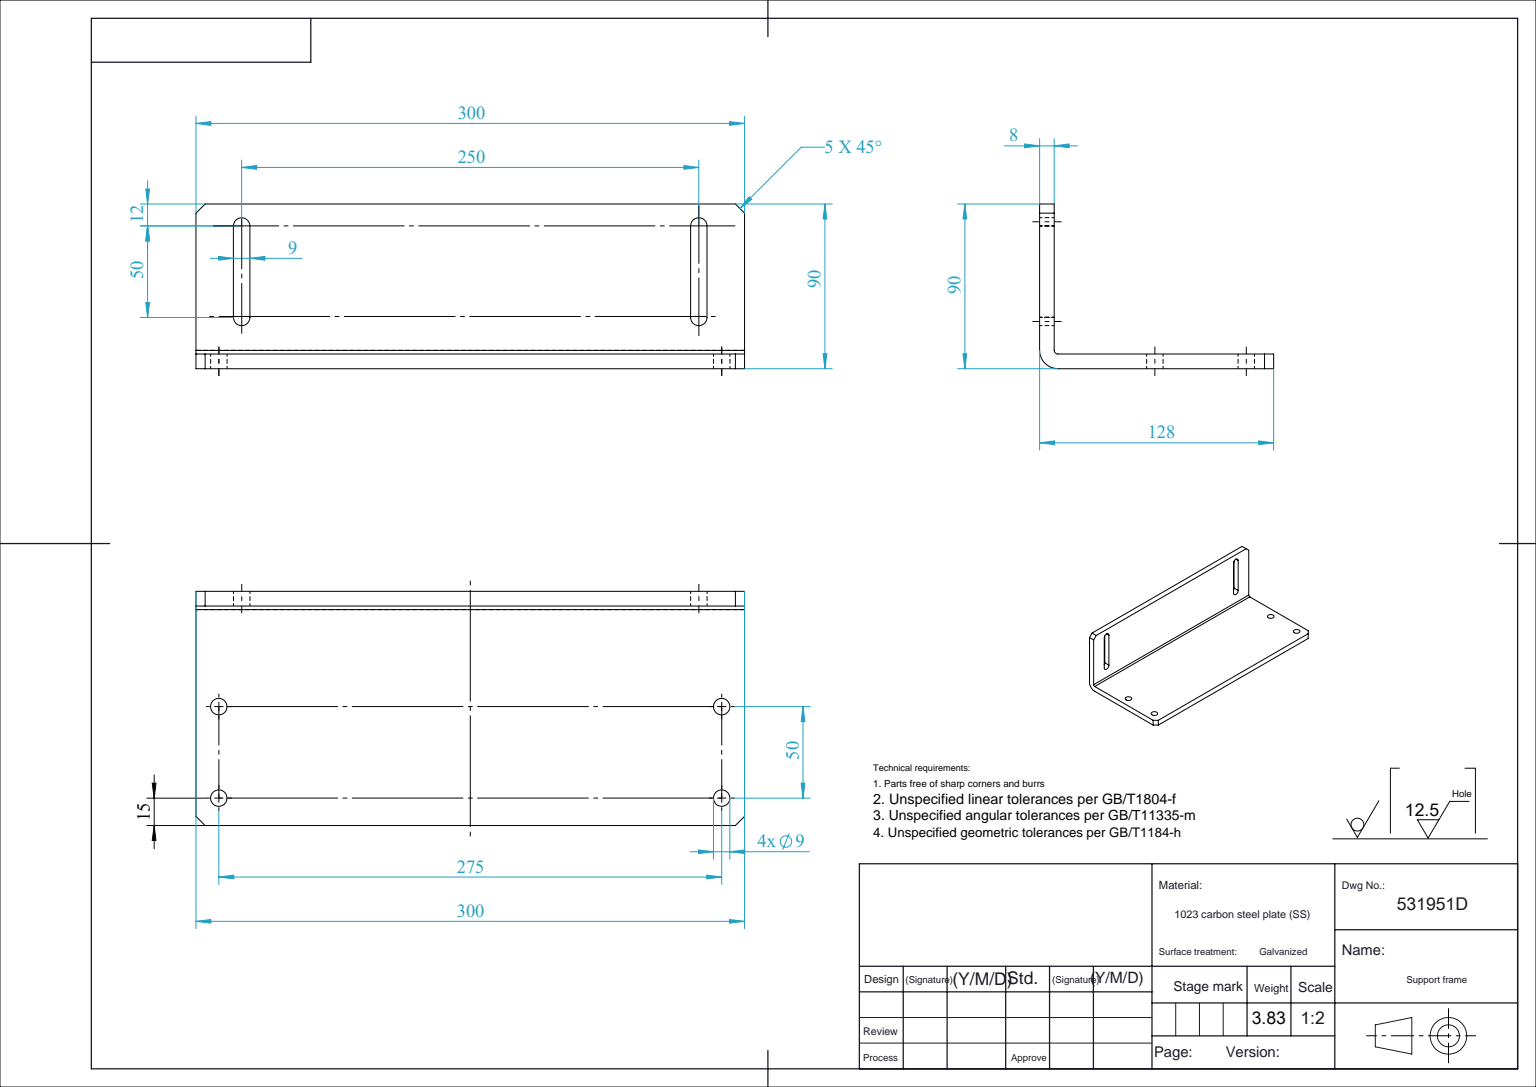
SolidWorks part; units mm, degrees
material "1023 carbon steel plate (SS)"
ref_plane "Front Plane" through (0, 0, 0) normal (0, 0, 1) x (1, 0, 0)
ref_plane "Top Plane" through (0, 0, 0) normal (0, 1, 0) x (1, 0, 0)
ref_plane "Right Plane" through (0, 0, 0) normal (1, 0, 0) x (0, 0, -1)
sketch "Sketch1" plane through (0, 0, 0) normal (0, 0, 1) x (1, 0, 0)
  line L0 (0, 0) -> (0, -90)
  line L1 (0, -90) -> (128, -90)
  line L2 (8, 0) -> (8, -82)
  line L3 (8, -82) -> (128, -82)
  line L4 (8, 0) -> (0, 0)
  line L5 (128, -82) -> (128, -90)
  dimension "D1" = 90
  dimension "D2" = 128
  dimension "D3" = 8
extrude "Boss-Extrude1" add sketch "Sketch1" along normal blind 300 contours L5 L1 L0 L4 L2 L3
sketch "Sketch2" plane through (0, -82, 0) normal (0, 1, 0) x (1, 0, 0)
  line L0 (8, -300) -> (128, -300) construction
  line L1 (128, -300) -> (128, 0) construction
  circle A0 centre (63, -12.5) radius 4.5
  circle A1 centre (113, -12.5) radius 4.5
  circle A2 centre (63, -287.5) radius 4.5
  circle A3 centre (113, -287.5) radius 4.5
  dimension "D3" = 9
  dimension "D4" = 50
  dimension "D5" = 15
  dimension "D1" = 275
  dimension "D2" = 12.5
extrude "Cut-Extrude1" cut sketch "Sketch2" against normal blind 300
sketch "Sketch3" plane through (8, 0, 0) normal (1, 0, 0) x (0, 0, -1)
  line L0 (-275, -12) -> (-275, -62) construction
  line L1 (-270.5, -12) -> (-270.5, -62)
  line L2 (-279.5, -12) -> (-279.5, -62)
  line L3 (-300, 0) -> (0, 0) construction
  line L4 (-300, 0) -> (-300, -82) construction
  line L5 (-150, 0) -> (-150, -47.7489) construction
  line L6 (-25, -12) -> (-25, -62) construction
  line L7 (-29.5, -12) -> (-29.5, -62)
  line L8 (-20.5, -12) -> (-20.5, -62)
  arc A0 (-270.5, -12) -> (-279.5, -12) centre (-275, -12) ccw
  arc A1 (-279.5, -62) -> (-270.5, -62) centre (-275, -62) ccw
  arc A2 (-29.5, -12) -> (-20.5, -12) centre (-25, -12) cw
  arc A3 (-20.5, -62) -> (-29.5, -62) centre (-25, -62) cw
  point P2 (-275, -37)
  point P15 (-25, -37)
  dimension "D1" = 4.5
  dimension "D2" = 12
  dimension "D3" = 50
  dimension "D4" = 25
extrude "Cut-Extrude2" cut sketch "Sketch3" against normal blind 300
chamfer "Chamfer1" distance 5 angle 45 4 edges at (128, -86, 300) (128, -86, 0) (4, 0, 0) (4, 0, 300)
fillet "Fillet1" radius 2 1 edges at (8, -82, 150)
fillet "Fillet2" radius 10 1 edges at (0, -90, 150)
